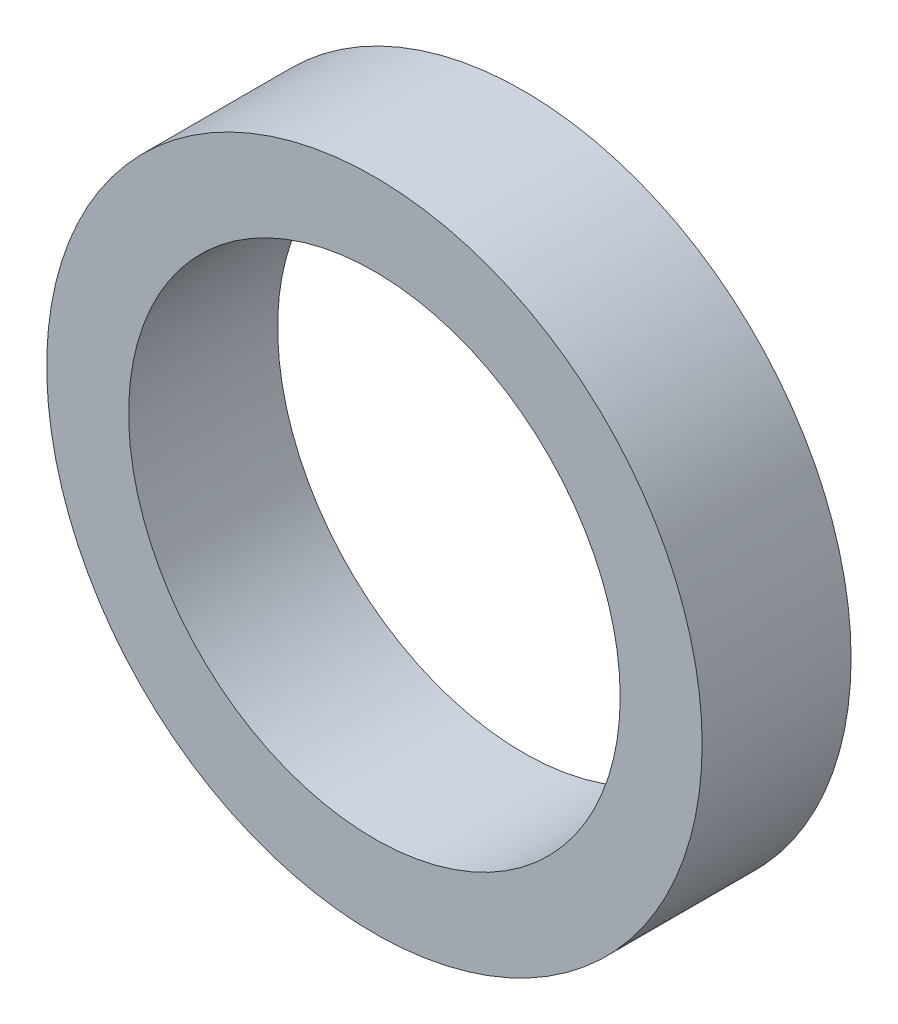
from build123d import *

# Parameters (mm, degrees)
SKETCH_1_R      = 11
SKETCH_1_R_2    = 8.25
EXTRUDE_1_DEPTH = 2.5


with BuildPart() as part:
    # 草图1 → 凸台-拉伸1 (new, symmetric)
    with BuildSketch(Plane.XY):
        Circle(SKETCH_1_R)
        Circle(SKETCH_1_R_2, mode=Mode.SUBTRACT)
    extrude(amount=EXTRUDE_1_DEPTH, both=True)


solid = part.part
